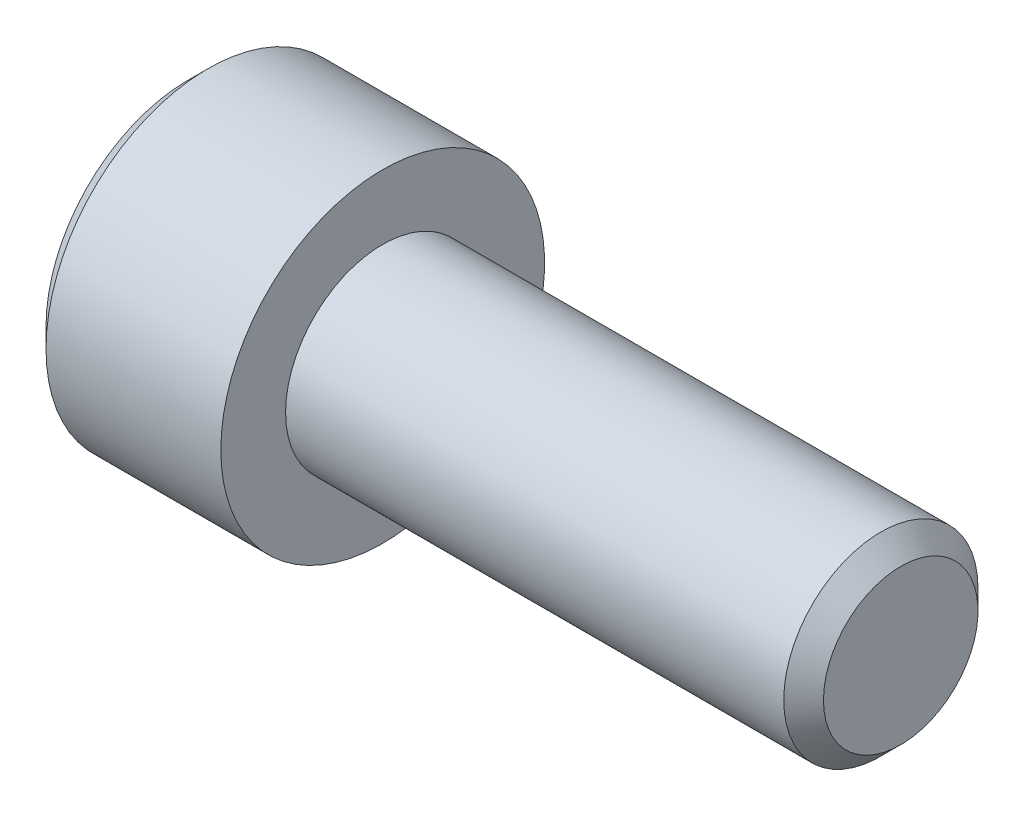
SolidWorks part; units mm, degrees
material "SUS304/0Cr18Ni9"
ref_plane "前视基准面" through (0, 0, 0) normal (0, 0, 1) x (1, 0, 0)
ref_plane "上视基准面" through (0, 0, 0) normal (0, 1, 0) x (1, 0, 0)
ref_plane "右视基准面" through (0, 0, 0) normal (1, 0, 0) x (0, 0, -1)
ref_plane "基准面4" through (0, 0, 0) normal (0, 0, 1) x (1, 0, 0)
sketch "草图1" plane through (0, 0, 0) normal (0, 0, 1) x (1, 0, 0)
  line L0 (-6, 0) -> (-6, 4.4)
  line L1 (-6, 4.4) -> (-5.4, 5)
  line L2 (-5.4, 5) -> (0, 5)
  line L3 (0, 5) -> (0, 3)
  line L4 (0, 3) -> (15.3865, 3)
  line L5 (15.3865, 3) -> (16, 2.3865)
  line L6 (16, 2.3865) -> (16, 0)
  line L7 (16, 0) -> (-6, 0)
  line L8 (16, 0) -> (-6, 0) construction
  dimension "D1" = 16
revolve "旋转1" add sketch "草图1" angle 360 about L8
ref_plane "基准面5" through (0, 0, 0) normal (0, 0, 1) x (1, 0, 0)
sketch "草图2" plane through (0, 0, 0) normal (0, 0, 1) x (1, 0, 0)
  line L0 (-6, 0) -> (-6, 2.5)
  line L1 (-6, 2.5) -> (-3, 2.5)
  line L2 (-3, 2.5) -> (-2.3301, 0)
  line L3 (-2.3301, 0) -> (-6, 0)
  line L4 (-2.3301, 0) -> (-6, 0) construction
revolve "切除-旋转1" cut sketch "草图2" angle 360 about L4
ref_plane "基准面6" through (-6, 0, 0) normal (1, 0, 0) x (0, 0, -1)
sketch "草图3" plane through (-6, 0, 0) normal (1, 0, 0) x (0, 0, -1)
  line L0 (-2.5, 1.4434) -> (-2.5, -1.4434)
  line L1 (-2.5, -1.4434) -> (0, -2.8868)
  line L2 (0, -2.8868) -> (2.5, -1.4434)
  line L3 (2.5, -1.4434) -> (2.5, 1.4434)
  line L4 (2.5, 1.4434) -> (0, 2.8868)
  line L5 (0, 2.8868) -> (-2.5, 1.4434)
extrude "切除-拉伸1" cut sketch "草图3" along normal blind 3
